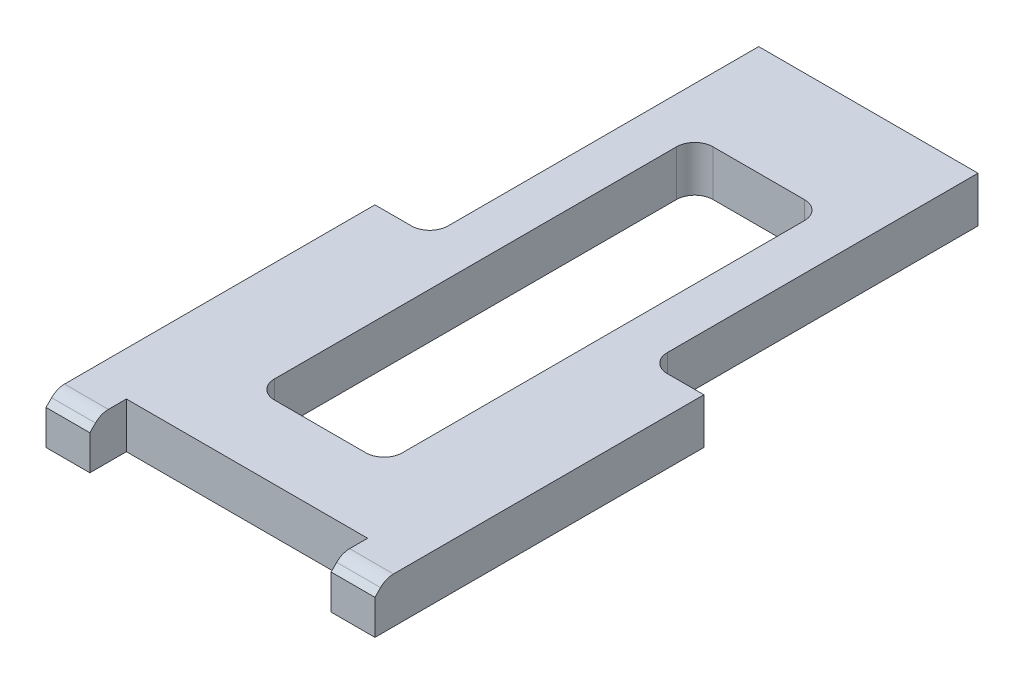
SolidWorks part; units mm, degrees
ref_plane "Front Plane" through (0, 0, 0) normal (0, 0, 1) x (1, 0, 0)
ref_plane "Top Plane" through (0, 0, 0) normal (0, 1, 0) x (1, 0, 0)
ref_plane "Right Plane" through (0, 0, 0) normal (1, 0, 0) x (0, 0, -1)
sketch "Sketch1" plane through (0, 0, 0) normal (0, 0, 1) x (1, 0, 0)
  line L0 (-45, 6.25) -> (45, -6.25) construction
  line L1 (-45, 6.25) -> (45, 6.25)
  line L2 (-45, 6.25) -> (-45, -6.25)
  line L3 (-45, -6.25) -> (45, -6.25)
  line L4 (45, 6.25) -> (45, -6.25)
  dimension "D1" = 12.5
  dimension "D2" = 90
extrude "Boss-Extrude1" add sketch "Sketch1" along normal blind 180
sketch "Sketch2" plane through (0, 6.25, 0) normal (0, 1, 0) x (1, 0, 0)
  line L0 (45, -180) -> (-45, -180) construction
  line L1 (33, -180) -> (-33, -180)
  line L2 (33, -180) -> (33, -170)
  line L3 (33, -170) -> (-33, -170)
  line L4 (-33, -180) -> (-33, -170)
  line L5 (0, 0) -> (0, -170) construction
  line L6 (45, 0) -> (-45, 0) construction
  line L7 (-45, -180) -> (-45, 0) construction
  dimension "D1" = 10
  dimension "D2" = 12
extrude "Cut-Extrude1" cut sketch "Sketch2" against normal through all
chamfer "Chamfer1" distance 3 angle 45 2 edges at (-39, 6.25, 180) (39, 6.25, 180)
fillet "Fillet1" radius 5 2 edges at (-39, 6.25, 177) (39, 6.25, 177)
sketch "Sketch3" plane through (0, 6.25, 0) normal (0, 1, 0) x (1, 0, 0)
  line L0 (-45, -174.9289) -> (-45, 0) construction
  line L1 (45, 0) -> (30, 0)
  line L2 (45, 0) -> (45, -90)
  line L3 (45, -90) -> (30, -90)
  line L4 (30, 0) -> (30, -90)
  line L5 (-45, -90) -> (-30, -90)
  line L6 (-45, -90) -> (-45, 0)
  line L7 (-45, 0) -> (-30, 0)
  line L8 (-30, -90) -> (-30, 0)
  line L9 (45, 0) -> (-45, 0) construction
  dimension "D1" = 60
  dimension "D2" = 90
extrude "Cut-Extrude2" cut sketch "Sketch3" against normal through all
sketch "Sketch4" plane through (0, 6.25, 0) normal (0, 1, 0) x (1, 0, 0)
  line L0 (0, -30) -> (0, 0) construction
  line L1 (-17.5, -150) -> (17.5, -150)
  line L2 (-17.5, -150) -> (-17.5, -30)
  line L3 (-17.5, -30) -> (17.5, -30)
  line L4 (17.5, -150) -> (17.5, -30)
  line L5 (30, 0) -> (-30, 0) construction
  line L6 (33, -170) -> (-33, -170) construction
  dimension "D1" = 30
  dimension "D2" = 35
  dimension "D3" = 20
extrude "Cut-Extrude3" cut sketch "Sketch4" against normal through all
fillet "Fillet2" radius 5 4 edges at (17.5, 0, 30) (-17.5, 0, 30) (17.5, 0, 150) (-17.5, 0, 150)
fillet "Fillet3" radius 5 2 edges at (-30, 0, 90) (30, 0, 90)
